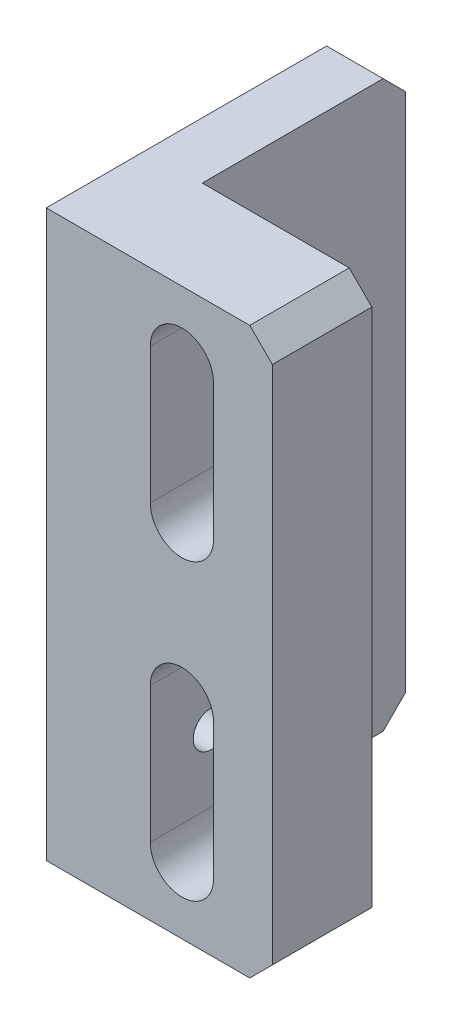
SolidWorks part; units mm, degrees
ref_plane "Front Plane" through (0, 0, 0) normal (0, 0, 1) x (1, 0, 0)
ref_plane "Top Plane" through (0, 0, 0) normal (0, 1, 0) x (1, 0, 0)
ref_plane "Right Plane" through (0, 0, 0) normal (1, 0, 0) x (0, 0, -1)
sketch "Sketch1" plane through (0, 0, 0) normal (0, 1, 0) x (1, 0, 0)
  line L1 (0, 0) -> (10, 0)
  line L2 (0, 0) -> (0, 13.4)
  line L3 (0, 13.4) -> (10, 13.4)
  line L4 (10, 0) -> (10, 13.4)
  dimension "D1" = 13.4
  dimension "D4" = 10
extrude "Boss-Extrude1" add sketch "Sketch1" along normal blind 25
sketch "Q" plane through (0, 0, 0) normal (0, 0, 1) x (1, 0, 0)
  line L0 (0, 12.5) -> (50000, 12.5) construction
  line L1 (0, 25) -> (0, 0) construction
  line L2 (6, 22) -> (6, 16) construction
  line L3 (7.4, 22) -> (7.4, 16)
  line L4 (4.6, 22) -> (4.6, 16)
  line L5 (6, 3) -> (6, 9) construction
  line L6 (7.4, 3) -> (7.4, 9)
  line L7 (4.6, 3) -> (4.6, 9)
  line L8 (10, 25) -> (10, 0) construction
  arc A0 (7.4, 22) -> (4.6, 22) centre (6, 22) ccw
  arc A1 (4.6, 16) -> (7.4, 16) centre (6, 16) ccw
  arc A2 (7.4, 3) -> (4.6, 3) centre (6, 3) cw
  arc A3 (4.6, 9) -> (7.4, 9) centre (6, 9) cw
  point P4 (0, 12.5)
  point P7 (6, 19)
  point P14 (6, 6)
  dimension "D1" = 2.8
  dimension "D2" = 13
  dimension "D3" = 6
  dimension "D4" = 4
extrude "Cut-Extrude2" cut sketch "Q" against normal blind 14
hole_wizard "M2 Tapped Hole1" positions "Sketch6" profile "Sketch5" tap size "M2" standard "Gb"
sketch "Sketch6" plane through (0, 0, 0) normal (-1, 0, 0) x (0, 0, 1)
  line L0 (-13.4, 25) -> (-13.4, 0) construction
  line L1 (-13.4, 0) -> (0, 0) construction
  point P0 (-10.7, 6)
  point P3 (-2.7, 6)
  dimension "D1" = 8
  dimension "D2" = 2.7
  dimension "D3" = 6
sketch "Sketch5" plane through (0, 6, -10.7) normal (0, 1, 0) x (0, 0, 1)
  line L0 (0, 0) -> (0, 5.6807)
  line L1 (0, 5.6807) -> (0.8, 5.2)
  line L2 (0.8, 5.2) -> (0.8, 0)
  line L5 (0.8, 0) -> (0, 0)
  line L10 (0, 5.6807) -> (-0.8, 5.2) construction
  line L11 (0, -6.35) -> (0, 107.95) construction
  dimension "螺纹孔钻头直径" = 1.6
  dimension "螺纹孔钻头深度" = 5.2
  dimension "导头角度" = 118
cosmetic thread "Cosmetic Thread1" parameters "D1"=4, "D2"=2
cosmetic thread "Cosmetic Thread2" parameters "D1"=4, "D2"=2
sketch "Sketch7" plane through (0, 0, -13.4) normal (0, 0, -1) x (-1, 0, 0)
  line L0 (-10, 25) -> (0, 25) construction
  line L1 (-2.5, 25) -> (-12.0638, 25)
  line L2 (-2.5, 25) -> (-2.5, 0)
  line L3 (-2.5, 0) -> (-12.0638, 0)
  line L4 (-12.0638, 25) -> (-12.0638, 0)
  arc A0 (-4.6, 9) -> (-7.4, 9) centre (-6, 9) ccw construction
  dimension "D1" = 3.5
extrude "Cut-Extrude3" cut sketch "Sketch7" against normal blind 9
chamfer "Chamfer1" distance 1 angle 45 6 edges at (10, 0, -2.2) (10, 25, -2.2) (1.25, 25, -13.4) (1.25, 0, -13.4) (0, 0, -6.7) (0, 25, -6.7)
